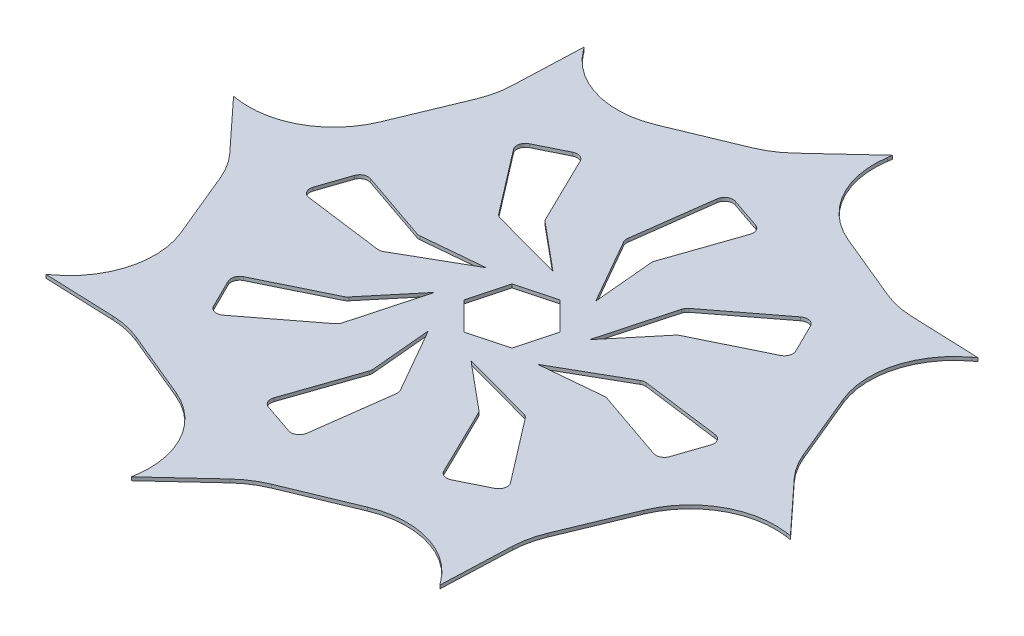
from build123d import *

# Parameters (mm, degrees)
BOSS_EXTRUDE1_DEPTH = 2
CUT_EXTRUDE1_DEPTH  = 10
CUT_EXTRUDE2_DEPTH  = 10
BOSS_EXTRUDE2_DEPTH = 2
FILLET1_R           = 50


with BuildPart() as part:
    # Sketch1 → Boss-Extrude1 (new body)
    with BuildSketch(Plane(origin=(0, 0, 0), x_dir=(1, 0, 0), z_dir=(0, 1, 0))):
        Polygon((114.80502971, -114.80502971), (162.358830044, 0), (114.80502971, 114.80502971), (0, 162.358830044), (-114.80502971, 114.80502971), (-162.358830044, 0), (-114.80502971, -114.80502971), (0, -162.358830044), align=None)
    extrude(amount=BOSS_EXTRUDE1_DEPTH)

    # Sketch2 → Cut-Extrude1 (cut)
    with BuildSketch(Plane(origin=(0, 2, 0), x_dir=(1, 0, 0), z_dir=(0, 1, 0))):
        Polygon((5.977169814, 22.307101433), (-16.329931619, 16.329931619), (-22.307101433, -5.977169814), (-5.977169814, -22.307101433), (16.329931619, -16.329931619), (22.307101433, 5.977169814), align=None)
    extrude(amount=-CUT_EXTRUDE1_DEPTH, mode=Mode.SUBTRACT)

    # Sketch3 → Cut-Extrude2 (cut)
    with BuildSketch(Plane(origin=(0, 2, 0), x_dir=(1, 0, 0), z_dir=(0, 1, 0))):
        with BuildLine():
            Line((7.180747689, 123.974968015), (25.207285, 117.858821427))
            ThreePointArc((25.207285, 117.858821427), (28.089576698, 115.326406795), (28.328747659, 111.497108353))
            Line((28.328747659, 111.497108353), (13.99872444, 69.850478373))
            ThreePointArc((13.99872444, 69.850478373), (13.762569524, 68.82175425), (13.747623306, 67.766377979))
            Line((13.747623306, 67.766377979), (17.02042887, 32.130840461))
            Line((17.02042887, 32.130840461), (-4.884764675, 70.429589412))
            ThreePointArc((-4.884764675, 70.429589412), (-5.450629901, 71.947522663), (-5.501487679, 73.566700941))
            Line((-5.501487679, 73.566700941), (0.617313414, 119.89476636))
            ThreePointArc((0.617313414, 119.89476636), (2.934488498, 123.486434711), (7.180747689, 123.974968015))
        make_face()
        with BuildLine():
            Line((92.741095966, 82.585985196), (101.163014013, 65.514529695))
            ThreePointArc((101.163014013, 65.514529695), (101.410414459, 61.68575413), (98.871810971, 58.808911827))
            Line((98.871810971, 58.808911827), (59.290339906, 39.493153947))
            ThreePointArc((59.290339906, 39.493153947), (58.395935361, 38.932722886), (57.63910307, 38.197027741))
            Line((57.63910307, 38.197027741), (34.755195848, 10.684674503))
            Line((34.755195848, 10.684674503), (46.347190043, 53.255290495))
            ThreePointArc((46.347190043, 53.255290495), (47.0204038, 54.72875853), (48.129373861, 55.909652349))
            Line((48.129373861, 55.909652349), (85.214908823, 84.34189582))
            ThreePointArc((85.214908823, 84.34189582), (89.393092084, 85.243098653), (92.741095966, 82.585985196))
        make_face()
        with BuildLine():
            Line((123.974968015, -7.180747689), (117.858821427, -25.207285))
            ThreePointArc((117.858821427, -25.207285), (115.326406795, -28.089576698), (111.497108353, -28.328747659))
            Line((111.497108353, -28.328747659), (69.850478373, -13.99872444))
            ThreePointArc((69.850478373, -13.99872444), (68.82175425, -13.762569524), (67.766377979, -13.747623306))
            Line((67.766377979, -13.747623306), (32.130840461, -17.02042887))
            Line((32.130840461, -17.02042887), (70.429589412, 4.884764675))
            ThreePointArc((70.429589412, 4.884764675), (71.947522663, 5.450629901), (73.566700941, 5.501487679))
            Line((73.566700941, 5.501487679), (119.89476636, -0.617313414))
            ThreePointArc((119.89476636, -0.617313414), (123.486434711, -2.934488498), (123.974968015, -7.180747689))
        make_face()
        with BuildLine():
            Line((82.585985196, -92.741095966), (65.514529695, -101.163014013))
            ThreePointArc((65.514529695, -101.163014013), (61.68575413, -101.410414459), (58.808911827, -98.871810971))
            Line((58.808911827, -98.871810971), (39.493153947, -59.290339906))
            ThreePointArc((39.493153947, -59.290339906), (38.932722886, -58.395935361), (38.197027741, -57.63910307))
            Line((38.197027741, -57.63910307), (10.684674503, -34.755195848))
            Line((10.684674503, -34.755195848), (53.255290495, -46.347190043))
            ThreePointArc((53.255290495, -46.347190043), (54.72875853, -47.0204038), (55.909652349, -48.129373861))
            Line((55.909652349, -48.129373861), (84.34189582, -85.214908823))
            ThreePointArc((84.34189582, -85.214908823), (85.243098653, -89.393092084), (82.585985196, -92.741095966))
        make_face()
        with BuildLine():
            Line((-7.180747689, -123.974968015), (-25.207285, -117.858821427))
            ThreePointArc((-25.207285, -117.858821427), (-28.089576698, -115.326406795), (-28.328747659, -111.497108353))
            Line((-28.328747659, -111.497108353), (-13.99872444, -69.850478373))
            ThreePointArc((-13.99872444, -69.850478373), (-13.762569524, -68.82175425), (-13.747623306, -67.766377979))
            Line((-13.747623306, -67.766377979), (-17.02042887, -32.130840461))
            Line((-17.02042887, -32.130840461), (4.884764675, -70.429589412))
            ThreePointArc((4.884764675, -70.429589412), (5.450629901, -71.947522663), (5.501487679, -73.566700941))
            Line((5.501487679, -73.566700941), (-0.617313414, -119.89476636))
            ThreePointArc((-0.617313414, -119.89476636), (-2.934488497, -123.486434711), (-7.180747689, -123.974968015))
        make_face()
        with BuildLine():
            Line((-92.741095966, -82.585985196), (-101.163014013, -65.514529695))
            ThreePointArc((-101.163014013, -65.514529695), (-101.410414459, -61.68575413), (-98.871810971, -58.808911827))
            Line((-98.871810971, -58.808911827), (-59.290339906, -39.493153947))
            ThreePointArc((-59.290339906, -39.493153947), (-58.395935361, -38.932722886), (-57.63910307, -38.197027741))
            Line((-57.63910307, -38.197027741), (-34.755195848, -10.684674503))
            Line((-34.755195848, -10.684674503), (-46.347190043, -53.255290495))
            ThreePointArc((-46.347190043, -53.255290495), (-47.0204038, -54.72875853), (-48.129373861, -55.909652349))
            Line((-48.129373861, -55.909652349), (-85.214908823, -84.34189582))
            ThreePointArc((-85.214908823, -84.34189582), (-89.393092084, -85.243098653), (-92.741095966, -82.585985196))
        make_face()
        with BuildLine():
            Line((-123.974968015, 7.180747689), (-117.858821427, 25.207285))
            ThreePointArc((-117.858821427, 25.207285), (-115.326406795, 28.089576698), (-111.497108353, 28.328747659))
            Line((-111.497108353, 28.328747659), (-69.850478373, 13.99872444))
            ThreePointArc((-69.850478373, 13.99872444), (-68.82175425, 13.762569524), (-67.766377979, 13.747623306))
            Line((-67.766377979, 13.747623306), (-32.130840461, 17.02042887))
            Line((-32.130840461, 17.02042887), (-70.429589412, -4.884764675))
            ThreePointArc((-70.429589412, -4.884764675), (-71.947522663, -5.450629901), (-73.566700941, -5.501487679))
            Line((-73.566700941, -5.501487679), (-119.89476636, 0.617313414))
            ThreePointArc((-119.89476636, 0.617313414), (-123.486434711, 2.934488497), (-123.974968015, 7.180747689))
        make_face()
        with BuildLine():
            Line((-82.585985196, 92.741095966), (-65.514529695, 101.163014013))
            ThreePointArc((-65.514529695, 101.163014013), (-61.68575413, 101.410414459), (-58.808911827, 98.871810971))
            Line((-58.808911827, 98.871810971), (-39.493153947, 59.290339906))
            ThreePointArc((-39.493153947, 59.290339906), (-38.932722886, 58.395935361), (-38.197027741, 57.63910307))
            Line((-38.197027741, 57.63910307), (-10.684674503, 34.755195848))
            Line((-10.684674503, 34.755195848), (-53.255290495, 46.347190043))
            ThreePointArc((-53.255290495, 46.347190043), (-54.72875853, 47.0204038), (-55.909652349, 48.129373861))
            Line((-55.909652349, 48.129373861), (-84.34189582, 85.214908823))
            ThreePointArc((-84.34189582, 85.214908823), (-85.243098653, 89.393092084), (-82.585985196, 92.741095966))
        make_face()
    extrude(amount=-CUT_EXTRUDE2_DEPTH, mode=Mode.SUBTRACT)

    # Sketch6 → Boss-Extrude2 (add)
    with BuildSketch(Plane(origin=(0, 2, 0), x_dir=(1, 0, 0), z_dir=(0, 1, 0))):
        Polygon((-117.573883954, 108.120424241), (-115.657269767, 158.083676638), (-90.835857439, 124.733385943), (-114.80502971, 114.80502971), align=None)
        Polygon((-6.684605468, 159.5899758), (30, 193.564079491), (23.969172271, 152.43047381), (0, 162.358830044), align=None)
        Polygon((108.120424241, 117.573883954), (158.083676638, 115.657269767), (124.733385943, 90.835857439), (114.80502971, 114.80502971), align=None)
        Polygon((159.5899758, 6.684605468), (193.564079491, -30), (152.43047381, -23.969172271), (162.358830044, 0), align=None)
        Polygon((117.573883954, -108.120424241), (115.657269767, -158.083676638), (90.835857439, -124.733385943), (114.80502971, -114.80502971), align=None)
        Polygon((6.684605468, -159.5899758), (-30, -193.564079491), (-23.969172271, -152.43047381), (0, -162.358830044), align=None)
        Polygon((-108.120424241, -117.573883954), (-158.083676638, -115.657269767), (-124.733385943, -90.835857439), (-114.80502971, -114.80502971), align=None)
        Polygon((-159.5899758, -6.684605468), (-193.564079491, 30), (-152.43047381, 23.969172271), (-162.358830044, 0), align=None)
    extrude(amount=-BOSS_EXTRUDE2_DEPTH)

    # Fillet1
    fillet1_edges = [part.edges().sort_by_distance(p)[0] for p in [
        (-117.573883954, 1, -108.120424241),
        (-90.835857439, 1, -124.733385943),
        (-6.684605468, 1, -159.5899758),
        (23.969172271, 1, -152.43047381),
        (108.120424241, 1, -117.573883954),
        (124.733385943, 1, -90.835857439),
        (159.5899758, 1, -6.684605468),
        (152.43047381, 1, 23.969172271),
        (117.573883954, 1, 108.120424241),
        (90.835857439, 1, 124.733385943),
        (6.684605468, 1, 159.5899758),
        (-23.969172271, 1, 152.43047381),
        (-108.120424241, 1, 117.573883954),
        (-124.733385943, 1, 90.835857439),
        (-159.5899758, 1, 6.684605468),
        (-152.43047381, 1, -23.969172271),
    ]]
    fillet(fillet1_edges, radius=FILLET1_R)


solid = part.part
